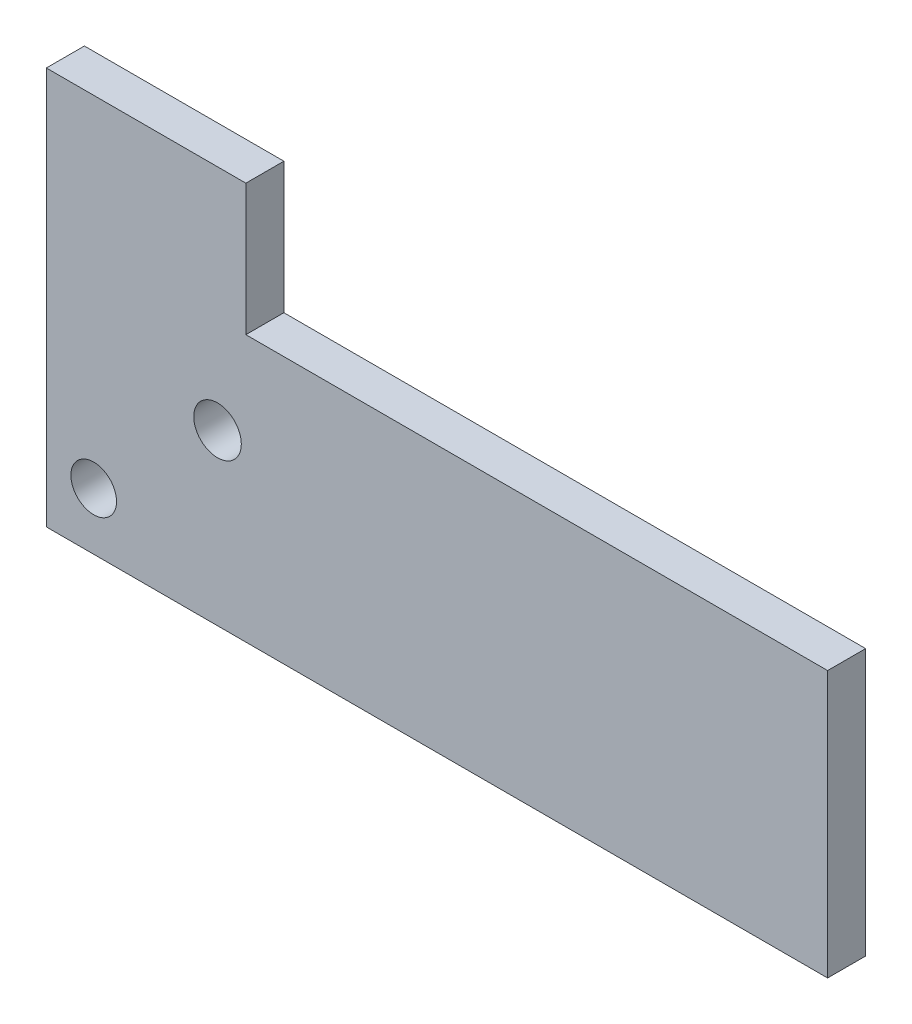
from build123d import *

# Parameters (mm, degrees)
SKETCH1_R           = 6
SKETCH1_R_2         = 6.25
BOSS_EXTRUDE1_DEPTH = 10


with BuildPart() as part:
    # Sketch1 → Boss-Extrude1 (new body)
    with BuildSketch(Plane.XY):
        Polygon((7.55, 34.5), (7.55, -70), (212.942105032, -70), (212.942105032, 0), (137.727272727, 0), (60, 0), (60, 34.5), align=None)
        with Locations((20, -55)):
            Circle(SKETCH1_R, mode=Mode.SUBTRACT)
        with Locations((52.55, -25.5)):
            Circle(SKETCH1_R_2, mode=Mode.SUBTRACT)
    extrude(amount=BOSS_EXTRUDE1_DEPTH)


solid = part.part
